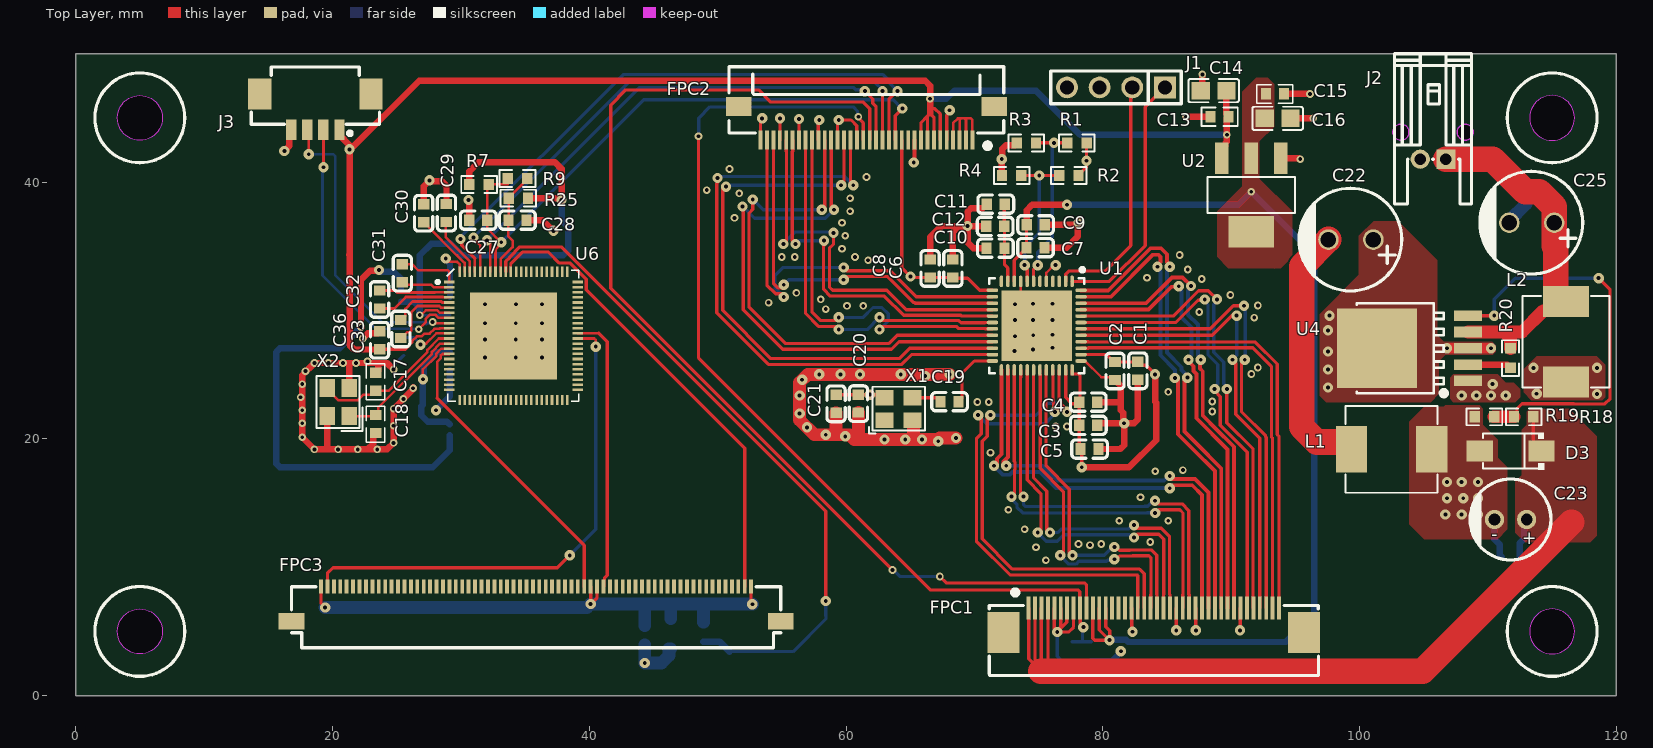
[diagram p0: Top Layer view]
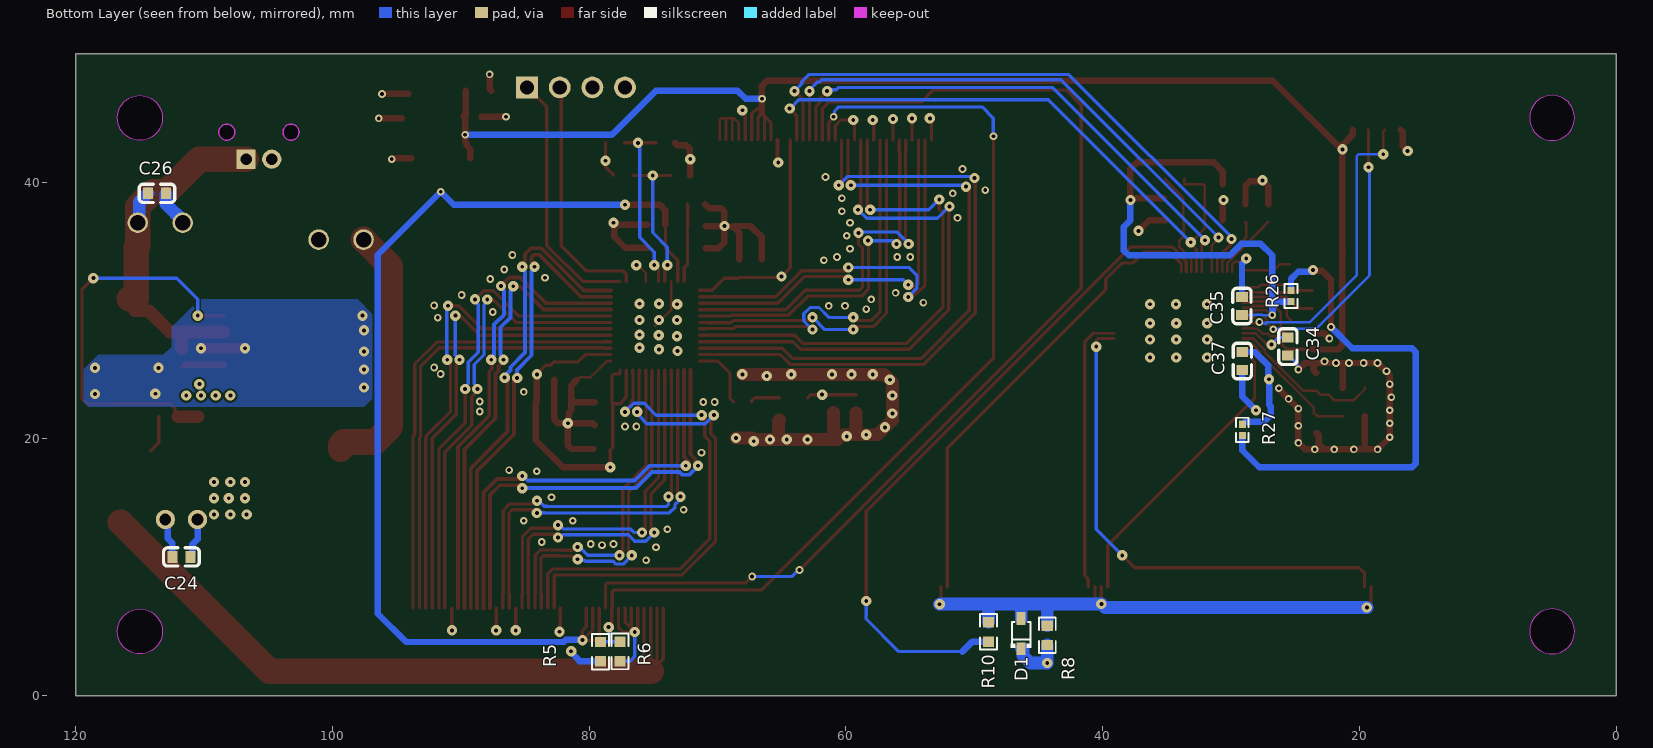
[diagram p1: Bottom Layer view, seen from below]
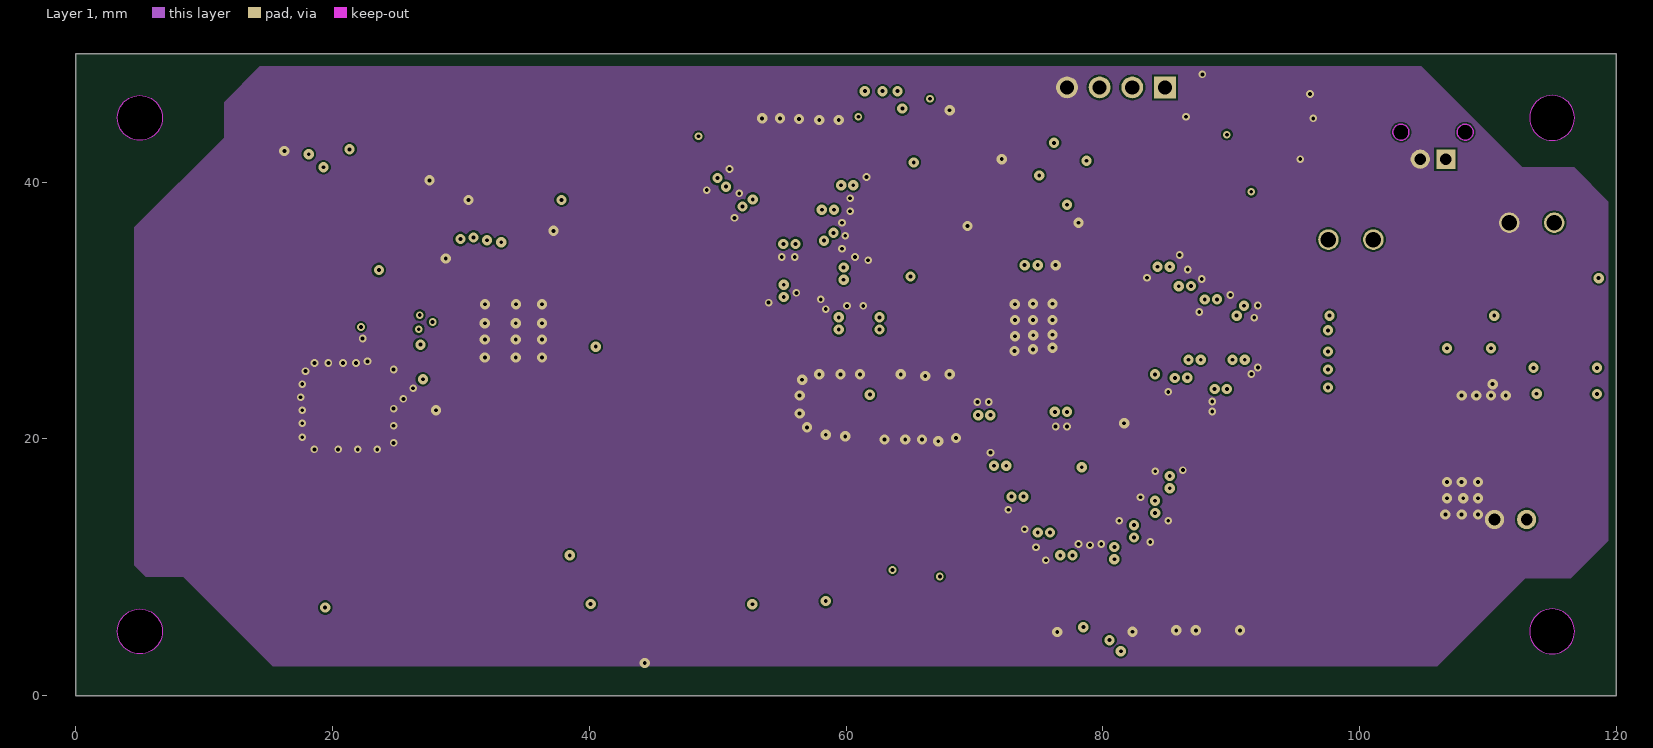
[diagram p2: Layer 1]
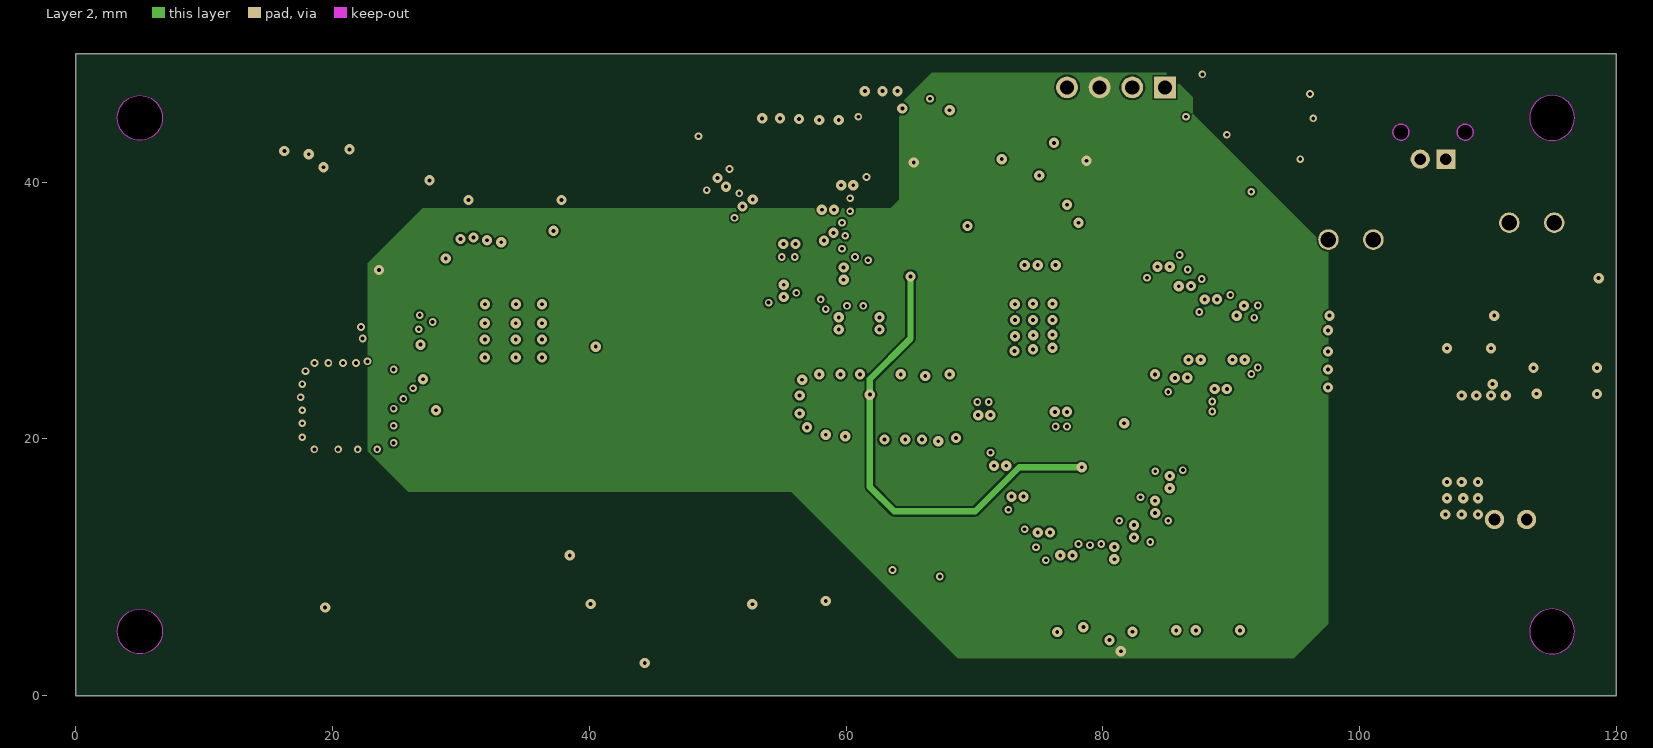
[diagram p3: Layer 2]
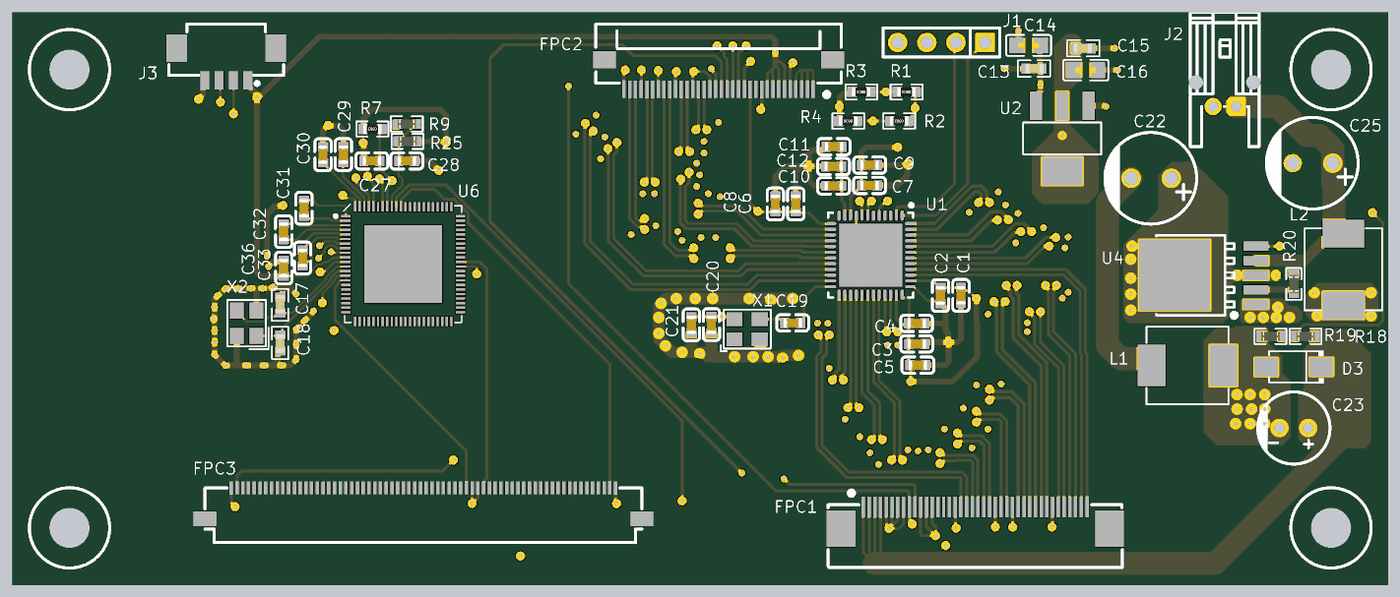
[diagram p4: 3D render of the assembled board from above, using the file's embedded part models]
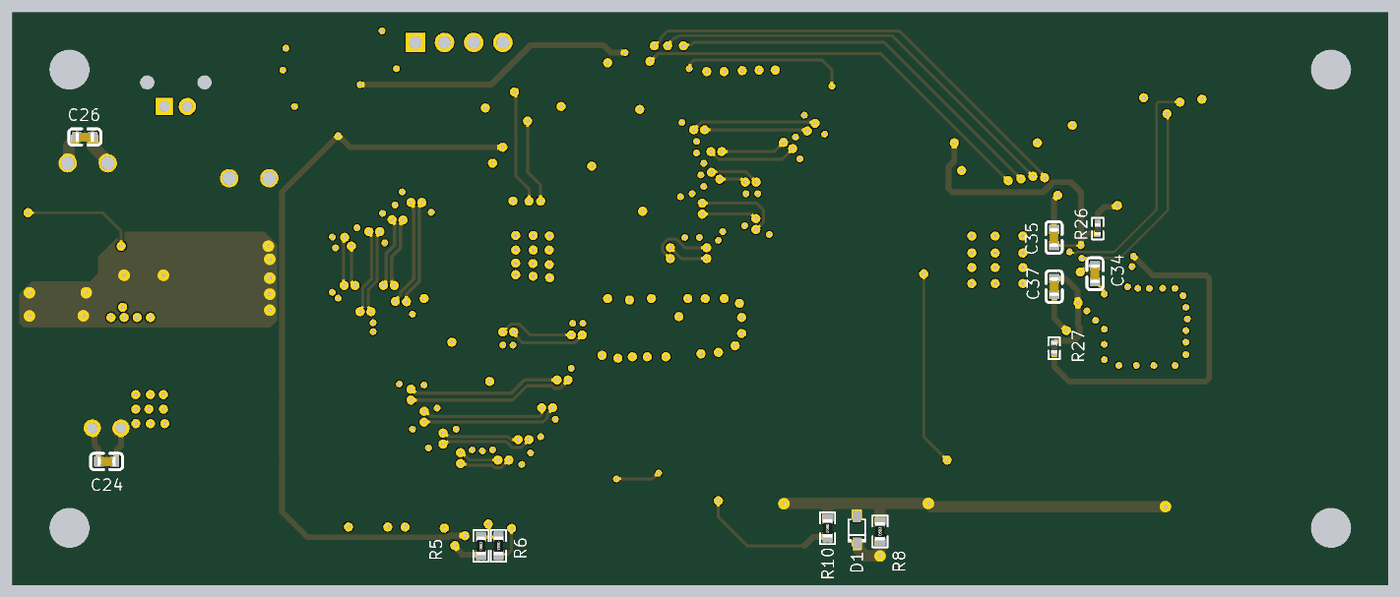
[diagram p5: 3D render of the assembled board from below, using the file's embedded part models]
# Altium PCB MISC71201-3.PcbDoc (part 1 of 3)
Units mm, origin at the board's own origin, x right, y up, seen from the top; angles counter-clockwise.
Board outline 120 x 50 mm, 4 copper layers (Top Layer, Layer 1, Layer 2, Bottom Layer), stack 0.603 mm thick; 69 components, 139 nets, 430 pads, 271 vias.

## Layer stack, top to bottom
Top Solder: solder mask 0.0102, Solder Resist, Dk 3.5
Top Layer: signal copper 0.0356
Dielectric 2: prepreg 0.0711, PP-006, Dk 4.1
Layer 1: signal copper 0.035
Dielectric 1: dielectric 0.32, FR-4, Dk 4.8
Layer 2: signal copper 0.035
Dielectric 3: prepreg 0.0711, PP-006, Dk 4.1
Bottom Layer: signal copper 0.0356
Bottom Solder: solder mask 0.0102, Solder Resist, Dk 3.5

## Board outline
0,0 120,0 120,50 0,50
cut-out: 113.25,45 ccw(c115,45) 115,43.25 ccw(c115,45) 116.75,45 ccw(c115,45) 115,46.75 ccw(c115,45)
cut-out: 113.25,5 ccw(c115,5) 115,3.25 ccw(c115,5) 116.75,5 ccw(c115,5) 115,6.75 ccw(c115,5)
cut-out: 5,3.25 cw(c5,5) 3.25,5 cw(c5,5) 5,6.75 cw(c5,5) 6.75,5 cw(c5,5)
cut-out: 5,43.25 cw(c5,45) 3.25,45 cw(c5,45) 5,46.75 cw(c5,45) 6.75,45 cw(c5,45)

## Design rules (kind name [scope] priority, off if disabled: settings)
Clearance [All] p1: gap=0.15 ignorepadtopadclearanceinfootprint=TRUE
ComponentClearance [All] p1: gap=0.01 collisioncheckmode=3 verticalgap=0.01 showdistances=FALSE
DiffPairsRouting DiffPairsRouting_14 [InDifferentialPair('MIPI_TD3')] p1: maxlimit=0.254 minlimit=0.2 mostfreqgap=0.2 toplayer_minwidth=0.15 toplayer_maxwidth=0.381 toplayer_prefwidth=0.3 midlayer1_minwidth=0.15 midlayer1_maxwidth=0.381 midlayer1_prefwidth=0.3 midlayer2_minwidth=0.15 midlayer2_maxwidth=0.381 midlayer2_prefwidth=0.3 bottomlayer_minwidth=0.15 bottomlayer_maxwidth=0.381 bottomlayer_prefwidth=0.3 maxuncoupledlength=12.7
DiffPairsRouting DiffPairsRouting_13 [InDifferentialPair('MIPI_TD2')] p2: maxlimit=0.254 minlimit=0.2 mostfreqgap=0.2 toplayer_minwidth=0.15 toplayer_maxwidth=0.381 toplayer_prefwidth=0.3 midlayer1_minwidth=0.15 midlayer1_maxwidth=0.381 midlayer1_prefwidth=0.3 midlayer2_minwidth=0.15 midlayer2_maxwidth=0.381 midlayer2_prefwidth=0.3 bottomlayer_minwidth=0.15 bottomlayer_maxwidth=0.381 bottomlayer_prefwidth=0.3 maxuncoupledlength=12.7
DiffPairsRouting DiffPairsRouting_12 [InDifferentialPair('MIPI_TD1')] p3: maxlimit=0.254 minlimit=0.2 mostfreqgap=0.2 toplayer_minwidth=0.15 toplayer_maxwidth=0.381 toplayer_prefwidth=0.3 midlayer1_minwidth=0.15 midlayer1_maxwidth=0.381 midlayer1_prefwidth=0.3 midlayer2_minwidth=0.15 midlayer2_maxwidth=0.381 midlayer2_prefwidth=0.3 bottomlayer_minwidth=0.15 bottomlayer_maxwidth=0.381 bottomlayer_prefwidth=0.3 maxuncoupledlength=12.7
DiffPairsRouting DiffPairsRouting_11 [InDifferentialPair('MIPI_TD0')] p4: maxlimit=0.254 minlimit=0.2 mostfreqgap=0.2 toplayer_minwidth=0.15 toplayer_maxwidth=0.381 toplayer_prefwidth=0.3 midlayer1_minwidth=0.15 midlayer1_maxwidth=0.381 midlayer1_prefwidth=0.3 midlayer2_minwidth=0.15 midlayer2_maxwidth=0.381 midlayer2_prefwidth=0.3 bottomlayer_minwidth=0.15 bottomlayer_maxwidth=0.381 bottomlayer_prefwidth=0.3 maxuncoupledlength=12.7
DiffPairsRouting DiffPairsRouting_10 [InDifferentialPair('MIPI_TC')] p5: maxlimit=0.254 minlimit=0.2 mostfreqgap=0.2 toplayer_minwidth=0.15 toplayer_maxwidth=0.381 toplayer_prefwidth=0.3 midlayer1_minwidth=0.15 midlayer1_maxwidth=0.381 midlayer1_prefwidth=0.3 midlayer2_minwidth=0.15 midlayer2_maxwidth=0.381 midlayer2_prefwidth=0.3 bottomlayer_minwidth=0.15 bottomlayer_maxwidth=0.381 bottomlayer_prefwidth=0.3 maxuncoupledlength=12.7
DiffPairsRouting DiffPairsRouting_9 [InDifferentialPair('RXOC')] p6: maxlimit=0.254 minlimit=0.2 mostfreqgap=0.2 toplayer_minwidth=0.15 toplayer_maxwidth=0.381 toplayer_prefwidth=0.3 midlayer1_minwidth=0.15 midlayer1_maxwidth=0.381 midlayer1_prefwidth=0.3 midlayer2_minwidth=0.15 midlayer2_maxwidth=0.381 midlayer2_prefwidth=0.3 bottomlayer_minwidth=0.15 bottomlayer_maxwidth=0.381 bottomlayer_prefwidth=0.3 maxuncoupledlength=12.7
DiffPairsRouting DiffPairsRouting_8 [InDifferentialPair('RXO3')] p7: maxlimit=0.254 minlimit=0.2 mostfreqgap=0.2 toplayer_minwidth=0.15 toplayer_maxwidth=0.381 toplayer_prefwidth=0.3 midlayer1_minwidth=0.15 midlayer1_maxwidth=0.381 midlayer1_prefwidth=0.3 midlayer2_minwidth=0.15 midlayer2_maxwidth=0.381 midlayer2_prefwidth=0.3 bottomlayer_minwidth=0.15 bottomlayer_maxwidth=0.381 bottomlayer_prefwidth=0.3 maxuncoupledlength=12.7
DiffPairsRouting DiffPairsRouting_7 [InDifferentialPair('RXO2')] p8: maxlimit=0.254 minlimit=0.2 mostfreqgap=0.2 toplayer_minwidth=0.15 toplayer_maxwidth=0.381 toplayer_prefwidth=0.3 midlayer1_minwidth=0.15 midlayer1_maxwidth=0.381 midlayer1_prefwidth=0.3 midlayer2_minwidth=0.15 midlayer2_maxwidth=0.381 midlayer2_prefwidth=0.3 bottomlayer_minwidth=0.15 bottomlayer_maxwidth=0.381 bottomlayer_prefwidth=0.3 maxuncoupledlength=12.7
DiffPairsRouting DiffPairsRouting_6 [InDifferentialPair('RXO1')] p9: maxlimit=0.254 minlimit=0.2 mostfreqgap=0.2 toplayer_minwidth=0.15 toplayer_maxwidth=0.381 toplayer_prefwidth=0.3 midlayer1_minwidth=0.15 midlayer1_maxwidth=0.381 midlayer1_prefwidth=0.3 midlayer2_minwidth=0.15 midlayer2_maxwidth=0.381 midlayer2_prefwidth=0.3 bottomlayer_minwidth=0.15 bottomlayer_maxwidth=0.381 bottomlayer_prefwidth=0.3 maxuncoupledlength=12.7
DiffPairsRouting DiffPairsRouting_5 [InDifferentialPair('RXO0')] p10: maxlimit=0.254 minlimit=0.2 mostfreqgap=0.2 toplayer_minwidth=0.15 toplayer_maxwidth=0.381 toplayer_prefwidth=0.3 midlayer1_minwidth=0.15 midlayer1_maxwidth=0.381 midlayer1_prefwidth=0.3 midlayer2_minwidth=0.15 midlayer2_maxwidth=0.381 midlayer2_prefwidth=0.3 bottomlayer_minwidth=0.15 bottomlayer_maxwidth=0.381 bottomlayer_prefwidth=0.3 maxuncoupledlength=12.7
DiffPairsRouting DiffPairsRouting_4 [InDifferentialPair('RXEC')] p11: maxlimit=0.254 minlimit=0.2 mostfreqgap=0.2 toplayer_minwidth=0.15 toplayer_maxwidth=0.381 toplayer_prefwidth=0.3 midlayer1_minwidth=0.15 midlayer1_maxwidth=0.381 midlayer1_prefwidth=0.3 midlayer2_minwidth=0.15 midlayer2_maxwidth=0.381 midlayer2_prefwidth=0.3 bottomlayer_minwidth=0.15 bottomlayer_maxwidth=0.381 bottomlayer_prefwidth=0.3 maxuncoupledlength=12.7
DiffPairsRouting DiffPairsRouting_3 [InDifferentialPair('RXE3')] p12: maxlimit=0.254 minlimit=0.2 mostfreqgap=0.2 toplayer_minwidth=0.15 toplayer_maxwidth=0.381 toplayer_prefwidth=0.3 midlayer1_minwidth=0.15 midlayer1_maxwidth=0.381 midlayer1_prefwidth=0.3 midlayer2_minwidth=0.15 midlayer2_maxwidth=0.381 midlayer2_prefwidth=0.3 bottomlayer_minwidth=0.15 bottomlayer_maxwidth=0.381 bottomlayer_prefwidth=0.3 maxuncoupledlength=12.7
DiffPairsRouting DiffPairsRouting_2 [InDifferentialPair('RXE2')] p13: maxlimit=0.254 minlimit=0.2 mostfreqgap=0.2 toplayer_minwidth=0.15 toplayer_maxwidth=0.381 toplayer_prefwidth=0.3 midlayer1_minwidth=0.15 midlayer1_maxwidth=0.381 midlayer1_prefwidth=0.3 midlayer2_minwidth=0.15 midlayer2_maxwidth=0.381 midlayer2_prefwidth=0.3 bottomlayer_minwidth=0.15 bottomlayer_maxwidth=0.381 bottomlayer_prefwidth=0.3 maxuncoupledlength=12.7
DiffPairsRouting DiffPairsRouting_1 [InDifferentialPair('RXE1')] p14: maxlimit=0.254 minlimit=0.2 mostfreqgap=0.2 toplayer_minwidth=0.15 toplayer_maxwidth=0.381 toplayer_prefwidth=0.3 midlayer1_minwidth=0.15 midlayer1_maxwidth=0.381 midlayer1_prefwidth=0.3 midlayer2_minwidth=0.15 midlayer2_maxwidth=0.381 midlayer2_prefwidth=0.3 bottomlayer_minwidth=0.15 bottomlayer_maxwidth=0.381 bottomlayer_prefwidth=0.3 maxuncoupledlength=12.7
DiffPairsRouting [InDifferentialPair('RXE0')] p15: maxlimit=0.254 minlimit=0.2 mostfreqgap=0.2 toplayer_minwidth=0.15 toplayer_maxwidth=0.3 toplayer_prefwidth=0.3 midlayer1_minwidth=0.15 midlayer1_maxwidth=0.3 midlayer1_prefwidth=0.3 midlayer2_minwidth=0.15 midlayer2_maxwidth=0.3 midlayer2_prefwidth=0.3 bottomlayer_minwidth=0.15 bottomlayer_maxwidth=0.3 bottomlayer_prefwidth=0.3 maxuncoupledlength=12.7
MinimumSolderMaskSliver [All] p1: minsoldermaskwidth=0.01
PlaneConnect [All] p1: planeconnectstyle=Direct reliefexpansion=0.508 reliefentries=4 reliefconductorwidth=0.254 reliefairgap=0.254
PolygonConnect [All] p1: connectstyle=Direct reliefconductorwidth=0.254 reliefentries=4 polygonreliefangle="90 Angle" airgapwidth=0.254
RoutingVias [All] p1: holewidth=0.3 width=0.8 viastyle="Through Hole" minholewidth=0.3 minwidth=0.8 maxholewidth=0.711 maxwidth=1.27
SilkToSilkClearance [All] p1: silktosilkclearance=0.01
SilkToSolderMaskClearance [IsPad] p1: minsilkscreentomaskgap=0.01 clearancetoexposedcopper=TRUE
SolderMaskExpansion [All] p1: expansion=0.102 istentingtop=FALSE
Width [All] p1: maxlimit=2 minlimit=0.18 preferedwidth=0.2
24 further rules are at their usual default settings.

## Classes and differential pairs
component class Sheet2: C17 C18 C27 C28 C29 C30 C31 C32 C33 C34 C35 C36 C37 D1 FPC3 J3 R7 R8 R9 R10 R25 R26 R27 U6 X2
component class Sheet1: C1 C2 C3 C4 C5 C6 C7 C8 C9 C10 C11 C12 C13 C14 C15 C16 C19 C20 C21 C22 C23 C24 C25 C26 D3 FPC1 FPC2 J1 J2 J? L1 L2 R1 R2 R3 R4 R5 R6 R18 R19 R20 U1 U2 U4 X1
differential pair MIPI_TD3: +MIPI_TD3_P -MIPI_TD3_N
differential pair MIPI_TD2: +MIPI_TD2_P -MIPI_TD2_N
differential pair MIPI_TD1: +MIPI_TD1_P -MIPI_TD1_N
differential pair MIPI_TD0: +MIPI_TD0_P -MIPI_TD0_N
differential pair MIPI_TC: +MIPI_TC_P -MIPI_TC_N
differential pair RXOC: +RXOC_P -RXOC_N
differential pair RXO3: +RXO3_P -RXO3_N
differential pair RXO2: +RXO2_P -RXO2_N
differential pair RXO1: +RXO1_P -RXO1_N
differential pair RXO0: +RXO0_P -RXO0_N
differential pair RXEC: +RXEC_P -RXEC_N
differential pair RXE3: +RXE3_P -RXE3_N
differential pair RXE2: +RXE2_P -RXE2_N
differential pair RXE1: +RXE1_P -RXE1_N
differential pair RXE0: +RXE0_P -RXE0_N

## Components (designator, comment, footprint, x,y, rotation, side; value= is the part's Value field where it differs from the comment)
C1 "cc0603krx7r0bb103" C0603 82.728,25.296 r90 top value=10nF
C2 "cc0603krx7r0bb103" C0603 80.95,25.281 r90 top value=10nF
C3 "cc0603krx7r0bb104" C0603 78.875,21.052 r180 top value=100nF
C4 "cc0603krx7r0bb104" C0603 78.869,22.85 r180 top value=100nF
C5 "cc0603krx7r8bb105" C0603 78.971,19.207 r0 top value=1uF
C6 "cc0603krx7r0bb103" C0603 68.326,33.274 r270 top value=10nF
C7 "cc0603krx7r0bb103" C0603 74.756,34.89 r180 top value=10nF
C8 "cc0603krx7r0bb104" C0603 66.548,33.274 r270 top value=100nF
C9 "cc0603krx7r0bb104" C0603 74.771,36.668 r180 top value=100nF
C10 "cc0603krx7r0bb103" C0603 71.636,34.851 r0 top value=10nF
C11 "cc0603krx7r0bb104" C0603 71.666,38.28 r0 top value=100nF
C12 "cc0603krx7r8bb105" C0603 71.62,36.546 r180 top value=1uF
C13 "100nF 50V 0603" "CAP C0603" 89.789,45.085 r180 top
C14 "10uF 25V 0805" "CAP C0805" 87.63,47.117 r0 top
C15 "100nF 50V 0603" "CAP C0603" 92.71,46.863 r0 top
C16 "10uF 25V 0805" "CAP C0805" 94.615,44.958 r180 top
C17 "CC0603JRNPO9BN120" "CAP C0603" 23.368,25.146 r270 top
C18 "CC0603JRNPO9BN120" "CAP C0603" 23.368,20.447 r90 top
C19 "cc0603krx7r9bb102" C0603 68.064,22.893 r180 top value=1nF
C20 "cc0603krx7r0bb103" C0603 60.97,22.741 r90 top value=10nF
C21 "cc0603krx7r0bb104" C0603 59.224,22.725 r90 top value=100nF
C22 "era63v100m8x12" CAP-TH_BD8.0-P3.50-D0.8-FD 99.325,35.518 r180 top value=100uF
C23 "erg25v220m6x11" CAP-TH_BD6.3-P2.50-D0.5-FD 111.76,13.716 r180 top value=220uF
C24 "cc0603krx7r0bb104" C0603 111.76,10.795 r0 bottom value=100nF
C25 "era63v100m8x12" CAP-TH_BD8.0-P3.50-D0.8-FD 113.411,36.83 r180 top value=100uF
C26 "cc0603krx7r0bb104" C0603 113.665,39.116 r0 bottom value=100nF
C27 "0.1u X7R 10% 6.3V" C0603 31.361,37.031 r180 top
C28 "2.2u X7R 10% 6.3V" C0603 34.409,37.031 r180 top
C29 "1u X7R 10% 50V" C0603 28.882,37.584 r270 top
C30 "1u X7R 10% 50V" C0603 27.104,37.569 r270 top
C31 "1u X7R 10% 50V" C0603 25.446,32.901 r270 top
C32 "1u X7R 10% 50V" C0603 23.675,30.853 r270 top
C33 "1u X7R 10% 50V" C0603 25.326,28.552 r270 top
C34 "1u X7R 10% 6.3V" C0603 25.58,27.186 r90 bottom
C35 "1u X7R 10% 6.3V" C0603 29.157,30.345 r270 bottom
C36 "1u X7R 10% 6.3V" C0603 23.675,27.678 r270 top
C37 "1u X7R 10% 6.3V" C0603 29.136,26.058 r90 bottom
D1 "pdyl240b" SOD-323_L1.8-W1.3-LS2.5-RD 46.355,4.826 r90 bottom
D3 "ss34" SMA_L4.3-W2.6-LS5.0-RD 111.76,19.05 r180 top
FPC1 "fc-05d40p11h20" FPC-SMD_40P-P0.50_FC-05D40P11H20 83.976,5.875 r0 top
FPC2 "fc-05a34p011h20" FPC-SMD_FC-05A34P011H20 61.595,44.577 r180 top
FPC3 "afc18-s68fia-00" CONN-SMD_AFC18-S68FIA-00 35.86,7.134 r0 top
J1 "hx pz2.54-1x4p zz" HDR-TH_4P-P2.54-V-M 81.026,47.371 r180 top
J2 "s02b-pask-2(lf)(sn)" CONN-TH_S02B-PASK-2-LF-SN 105.724,41.783 r0 top
J3 "mx1.25mm-4p-wt" CONN-SMD_MX1.25MM-4P-WT 18.669,45.466 r180 top
L1 "fxl0630-150-m" IND-SMD_L7.0-W6.6_FXL0630 102.489,19.177 r180 top
L2 "fxl0630-150-m" IND-SMD_L7.0-W6.6_FXL0630 116.078,27.559 r270 top
R1 "10K 0603 1%" "RES R0603" 78.74,43.053 r180 top
R2 "10K 0603 1%" "RES R0603" 78.105,40.513 r180 top
R3 "10K 0603 1%" "RES R0603" 74.803,43.053 r180 top
R4 "10K 0603 1%" "RES R0603" 73.66,40.513 r180 top
R5 "10K 0603 1%" "RES R0603" 79.121,2.667 r90 bottom
R6 "10K 0603 1%" "RES R0603" 77.597,4.191 r270 bottom
R7 "10K 0603 1% NC" "RES R0603" 32.171,39.818 r180 top
R8 "0R 0603" "RES R0603" 44.323,3.937 r90 bottom value=0R
R9 "0R 5% NC" R0603 34.417,40.259 r180 top value=10K
R10 "0R 0603" "RES R0603" 48.895,5.715 r270 bottom value=330R
R18 "rt0603brd0786k6l" R0603 112.776,21.717 r0 top value=86.6kΩ
R19 "rt0603brd0710kl" R0603 109.728,21.717 r180 top value=10kΩ
R20 "rt0603brd0710kl" R0603 111.76,26.289 r90 top value=10kΩ
R25 "0R 5%" R0603 34.478,38.738 r0 top value=10K
R26 "0R 5%" R0402 25.342,31.12 r270 bottom
R27 "0R 5%" R0402 29.134,20.696 r90 bottom
U1 "GM8775C" UFQFPN-48_L7.0-W7.0-P0.50-BL-EP 74.857,28.811 r180 top
U2 "bl1117-33cx" SOT-223_L6.5-W3.5-P2.30-LS7.0-BR 91.567,38.989 r90 top
U4 "xl6008e1" TO-252-5_L6.6-W5.8-P1.27-TL 104.902,27.051 r180 top
U6 "ILI2511/QFN-88/10X10" ILI2511/QFN-88/10X10 29.101,32.215 r0 top
X1 "ot322526mjba4sl" OSC-SMD_4P-L3.2-W2.5-BL 64.084,22.333 r0 top value=26MHz
X2 "x322512msb4si" CRYSTAL-SMD_4P-L3.2-W2.5-BL 20.447,22.86 r90 top value=12MHz

## Footprints (in the part's own frame and the unit in brackets; to place one, negate y for a bottom-side part, rotate by r counter-clockwise, add the part's x,y. Pads: shape width x height; smd on the part's side, far side on the other; paste and mask are expansions set on the pad)
C0603 [mil]
  rect 31.5x35.4 smd: 1(-27.5,0) 2(27.6,0)
  silkscreen extent -55,-28 55,28, body extent -31,-16 31,16, height 16
"CAP C0603" [mm]
  rect 0.8x0.9 smd: 1(0,0) 2(1.4,0)
  silkscreen extent -0.72,-0.72 2.1,0.72, body extent -0.17,-0.4 1.44,0.4, height 0.8
"CAP C0805" [mm]
  rect 1.41x1.35 smd paste-100 mask+0.051: 1(0,0) 2(2,0)
  silkscreen extent -0.96,-0.9 2.96,0.9, body extent 0.02,-0.63 2.02,0.63, height 0.6
CAP-TH_BD6.3-P2.50-D0.5-FD [mm]
  round 1.5 hole 0.9 paste-2539.97 mask+0.05: 1(-1.25,0) 2(1.25,0)
  silkscreen extent -3.15,-3.15 3.21,3.15
CAP-TH_BD8.0-P3.50-D0.8-FD [mm]
  round 1.6 hole 1.2 paste-2539.97 mask+0.05: 1(-1.75,0) 2(1.75,0)
  silkscreen extent -3.96,-4 4.04,4
CONN-SMD_AFC18-S68FIA-00 [mm]
  rect 0.3x1.1 smd paste+0 mask+0.05: 1(-16.75,1.35) 2(-16.25,1.35) 3(-15.75,1.35) 4(-15.25,1.35) 5(-14.75,1.35) 6(-14.25,1.35) 7(-13.75,1.35) 8(-13.25,1.35) 9(-12.75,1.35) 10(-12.25,1.35) 11(-11.75,1.35) 12(-11.25,1.35) 13(-10.75,1.35) 14(-10.25,1.35) 15(-9.75,1.35) 16(-9.25,1.35) 17(-8.75,1.35) 18(-8.25,1.35) 19(-7.75,1.35) 20(-7.25,1.35) 21(-6.75,1.35) 22(-6.25,1.35) 23(-5.75,1.35) 24(-5.25,1.35) 25(-4.75,1.35) 26(-4.25,1.35) 27(-3.75,1.35) 28(-3.25,1.35) 29(-2.75,1.35) 30(-2.25,1.35) 31(-1.75,1.35) 32(-1.25,1.35) 33(-0.75,1.35) 34(-0.25,1.35) 35(0.25,1.35) 36(0.75,1.35) 37(1.25,1.35) 38(1.75,1.35) 39(2.25,1.35) 40(2.75,1.35) 41(3.25,1.35) 42(3.75,1.35) 43(4.25,1.35) 44(4.75,1.35) 45(5.25,1.35) 46(5.75,1.35) 47(6.25,1.35) 48(6.75,1.35) 49(7.25,1.35) 50(7.75,1.35) 51(8.25,1.35) 52(8.75,1.35) 53(9.25,1.35) 54(9.75,1.35) 55(10.25,1.35) 56(10.75,1.35) 57(11.25,1.35) 58(11.75,1.35) 59(12.25,1.35) 60(12.75,1.35) 61(13.25,1.35) 62(13.75,1.35) 63(14.25,1.35) 64(14.75,1.35) 65(15.25,1.35) 66(15.75,1.35) 67(16.25,1.35) 68(16.75,1.35)
  rect 2x1.3 smd paste+0 mask+0.05: 69(19.05,-1.35) 70(-19.05,-1.35)
  silkscreen extent -19.05,-3.4 19.05,1.35
CONN-SMD_MX1.25MM-4P-WT [mm]
  rect 0.8x1.6 smd paste+0 mask+0.05: 1(-1.875,1.4) 2(-0.625,1.4) 3(0.625,1.4) 4(1.875,1.4)
  rect 1.8x2.4 smd paste+0 mask+0.05: 5(4.325,-1.4) 6(-4.325,-1.4)
  silkscreen extent -5,-3.5 5,1.82
CONN-TH_S02B-PASK-2-LF-SN [mm]
  rect 1.5x1.5 hole 0.9: 1(1,0)
  round 1.5 hole 0.9: 2(-1,0)
  Keep-Out Layer board cut-out: -1.875,2.1 -1.875,1.976 -1.97,1.746 -2.146,1.57 -2.376,1.475 -2.624,1.475 -2.854,1.57 -3.03,1.746 -3.125,1.976 -3.125,2.1 -3.125,2.224 -3.03,2.454 -2.854,2.63 -2.624,2.725 -2.376,2.725 -2.146,2.63 -1.97,2.454 -1.875,2.224 -1.875,2.1 -1.875,2.1
  Keep-Out Layer board cut-out: 3.125,2.1 3.125,1.976 3.03,1.746 2.854,1.57 2.624,1.475 2.376,1.475 2.146,1.57 1.97,1.746 1.875,1.976 1.875,2.1 1.875,2.224 1.97,2.454 2.146,2.63 2.376,2.725 2.624,2.725 2.854,2.63 3.03,2.454 3.125,2.224 3.125,2.1 3.125,2.1
  Keep-Out Layer circle w0.003: c-2.5,2.1 r0.625
  Keep-Out Layer circle w0.003: c2.5,2.1 r0.625
  Keep-Out Layer region: -1.875,2.1 -1.884,1.992 -1.913,1.886 -1.959,1.788 -2.021,1.698 -2.098,1.621 -2.187,1.559 -2.286,1.513 -2.391,1.485 -2.5,1.475 -2.608,1.485 -2.714,1.513 -2.812,1.559 -2.902,1.621 -2.979,1.698 -3.041,1.788 -3.087,1.886 -3.115,1.992 -3.125,2.1 -3.115,2.209 -3.087,2.314 -3.041,2.413 -2.979,2.502 -2.902,2.579 -2.812,2.641 -2.714,2.687 -2.608,2.716 -2.5,2.725 -2.391,2.716 -2.286,2.687 -2.187,2.641 -2.098,2.579 -2.021,2.502 -1.959,2.413 -1.913,2.314 -1.884,2.209 -1.875,2.1
  Keep-Out Layer region: -1.875,2.1 -1.875,1.976 -1.97,1.746 -2.146,1.57 -2.376,1.475 -2.624,1.475 -2.854,1.57 -3.03,1.746 -3.125,1.976 -3.125,2.1 -3.125,2.224 -3.03,2.454 -2.854,2.63 -2.624,2.725 -2.376,2.725 -2.146,2.63 -1.97,2.454 -1.875,2.224 -1.875,2.1 -1.875,2.1
  Keep-Out Layer region: 3.125,2.1 3.116,1.992 3.087,1.886 3.041,1.788 2.979,1.698 2.902,1.621 2.813,1.559 2.714,1.513 2.609,1.485 2.5,1.475 2.392,1.485 2.286,1.513 2.188,1.559 2.098,1.621 2.021,1.698 1.959,1.788 1.913,1.886 1.885,1.992 1.875,2.1 1.885,2.209 1.913,2.314 1.959,2.413 2.021,2.502 2.098,2.579 2.188,2.641 2.286,2.687 2.392,2.716 2.5,2.725 2.609,2.716 2.714,2.687 2.813,2.641 2.902,2.579 2.979,2.502 3.041,2.413 3.087,2.314 3.116,2.209 3.125,2.1
  Keep-Out Layer region: 3.125,2.1 3.125,1.976 3.03,1.746 2.854,1.57 2.624,1.475 2.376,1.475 2.146,1.57 1.97,1.746 1.875,1.976 1.875,2.1 1.875,2.224 1.97,2.454 2.146,2.63 2.376,2.725 2.624,2.725 2.854,2.63 3.03,2.454 3.125,2.224 3.125,2.1 3.125,2.1
  silkscreen extent -3,-3.5 3,8.2
CRYSTAL-SMD_4P-L3.2-W2.5-BL [mm]
  rect 1.4x1.2 smd: 1(-1.1,-0.85) 2(1.1,-0.85) 3(1.1,0.85) 4(-1.1,0.85)
  silkscreen extent -2.26,-1.91 2.03,1.68
FPC-SMD_40P-P0.50_FC-05D40P11H20 [mm]
  rect 0.3x1.8 smd paste+0 mask+0.05: 1(-9.75,0.95) 2(-9.25,0.95) 3(-8.75,0.95) 4(-8.25,0.95) 5(-7.75,0.95) 6(-7.25,0.95) 7(-6.75,0.95) 8(-6.25,0.95) 9(-5.75,0.95) 10(-5.25,0.95) 11(-4.75,0.95) 12(-4.25,0.95) 13(-3.75,0.95) 14(-3.25,0.95) 15(-2.75,0.95) 16(-2.25,0.95) 17(-1.75,0.95) 18(-1.25,0.95) 19(-0.75,0.95) 20(-0.25,0.95) 21(0.25,0.95) 22(0.75,0.95) 23(1.25,0.95) 24(1.75,0.95) 25(2.25,0.95) 26(2.75,0.95) 27(3.25,0.95) 28(3.75,0.95) 29(4.25,0.95) 30(4.75,0.95) 31(5.25,0.95) 32(5.75,0.95) 33(6.25,0.95) 34(6.75,0.95) 35(7.25,0.95) 36(7.75,0.95) 37(8.25,0.95) 38(8.75,0.95) 39(9.25,0.95) 40(9.75,0.95)
  rect 2.5x3.2 smd paste+0 mask+0.05: 41(11.7,-0.95) 42(-11.7,-0.95)
  silkscreen extent -12.83,-4.32 12.83,2.36
FPC-SMD_FC-05A34P011H20 [mm]
  rect 0.3x1.5 smd paste+0 mask+0.051: 1(8.25,1.3) 2(7.75,1.3) 3(7.25,1.3) 4(6.75,1.3) 5(6.25,1.3) 6(5.75,1.3) 7(5.25,1.3) 8(4.75,1.3) 9(4.25,1.3) 10(3.75,1.3) 11(3.25,1.3) 12(2.75,1.3) 13(2.25,1.3) 14(1.75,1.3) 15(1.25,1.3) 16(0.75,1.3) 17(0.25,1.3) 18(-0.25,1.3) 19(-0.75,1.3) 20(-1.25,1.3) 21(-1.75,1.3) 22(-2.25,1.3) 23(-2.75,1.3) 24(-3.25,1.3) 25(-3.75,1.3) 26(-4.25,1.3) 27(-4.75,1.3) 28(-5.25,1.3) 29(-5.75,1.3) 30(-6.25,1.3) 31(-6.75,1.3) 32(-7.25,1.3) 33(-7.75,1.3) 34(-8.25,1.3)
  rect 2x1.5 smd paste+0 mask+0.051: 35(9.95,-1.3) 36(-9.95,-1.3)
  silkscreen extent -10.7,-4.4 10.7,2.16
HDR-TH_4P-P2.54-V-M [mm]
  rect 1.699x1.699 hole 1.1: 1(-3.81,0)
  round 1.699 hole 1.1: 2(-1.27,0) 3(1.27,0) 4(3.81,0)
  silkscreen extent -5.08,-1.27 5.08,1.27
ILI2511/QFN-88/10X10 [mm]
  rect 0.8x0.2 smd: 1(0,0) 2(0,-0.4) 3(0,-0.8) 4(0,-1.2) 5(0,-1.6) 6(0,-2) 7(0,-2.4) 8(0,-2.8) 9(0,-3.2) 10(0,-3.6) 11(0,-4) 12(0,-4.4) 13(0,-4.8) 14(0,-5.2) 15(0,-5.6) 16(0,-6) 17(0,-6.4) 18(0,-6.8) 19(0,-7.2) 20(0,-7.6) 21(0,-8) 22(0,-8.4) 45(10,-8.4) 46(10,-8) 47(10,-7.6) 48(10,-7.2) 49(10,-6.8) 50(10,-6.4) 51(10,-6) 52(10,-5.6) 53(10,-5.2) 54(10,-4.8) 55(10,-4.4) 56(10,-4) 57(10,-3.6) 58(10,-3.2) 59(10,-2.8) 60(10,-2.4) 61(10,-2) 62(10,-1.6) 63(10,-1.2) 64(10,-0.8) 65(10,-0.4) 66(10,0)
  rect 0.2x0.8 smd: 23(0.8,-9.2) 24(1.2,-9.2) 25(1.6,-9.2) 26(2,-9.2) 27(2.4,-9.2) 28(2.8,-9.2) 29(3.2,-9.2) 30(3.6,-9.2) 31(4,-9.2) 32(4.4,-9.2) 33(4.8,-9.2) 34(5.2,-9.2) 35(5.6,-9.2) 36(6,-9.2) 37(6.4,-9.2) 38(6.8,-9.2) 39(7.2,-9.2) 40(7.6,-9.2) 41(8,-9.2) 42(8.4,-9.2) 43(8.8,-9.2) 44(9.2,-9.2) 67(9.2,0.8) 68(8.8,0.8) 69(8.4,0.8) 70(8,0.8) 71(7.6,0.8) 72(7.2,0.8) 73(6.8,0.8) 74(6.4,0.8) 75(6,0.8) 76(5.6,0.8) 77(5.2,0.8) 78(4.8,0.8) 79(4.4,0.8) 80(4,0.8) 81(3.6,0.8) 82(3.2,0.8) 83(2.8,0.8) 84(2.4,0.8) 85(2,0.8) 86(1.6,0.8) 87(1.2,0.8) 88(0.8,0.8)
  rect 6.8x6.8 smd: 89(5,-4.2)
  silkscreen extent -1.02,-9.3 10.1,1.03
IND-SMD_L7.0-W6.6_FXL0630 [mm]
  rect 2.424x3.62 smd: 1(3.128,0) 2(-3.128,0)
  silkscreen extent -3.58,-3.38 3.58,3.38
OSC-SMD_4P-L3.2-W2.5-BL [mm]
  rect 1.4x1.2 smd: 1(-1.1,-0.875) 2(1.1,-0.875) 3(1.1,0.875) 4(-1.1,0.875)
  silkscreen extent -2.29,-1.9 2.07,1.72
R0402 [mil]
  rect 22.3x21.3 smd paste-3937 mask+2: 1(-17.1,0) 2(17,0)
  silkscreen extent -37,-20 37,20, body extent -19,-10 23,10, height 28
R0603 [mil]
  rect 31.8x34 smd: 1(-29.6,0) 2(29.7,0)
  silkscreen extent -54,-26 55,26, body extent -32,-16 32,16, height 17
"RES R0603" [mm]
  rect 0.806x0.864 smd paste-100: 1(0,0) 2(1.507,0)
  silkscreen extent -0.63,-0.66 2.14,0.66, body extent -0.04,-0.4 1.56,0.4, height 0.43
SMA_L4.3-W2.6-LS5.0-RD [mm]
  rect 2.047x1.621 smd: 1(-2.403,-0.01) 2(2.405,0.01)
  silkscreen extent -2.61,-1.44 2.17,1.44
SOD-323_L1.8-W1.3-LS2.5-RD [mm]
  rect 1.001x0.701 smd: 1(-1.171,0) 2(1.173,0)
  silkscreen extent -1.08,-0.8 0.9,0.8
SOT-223_L6.5-W3.5-P2.30-LS7.0-BR [mm]
  rect 2.465x1.05 smd: 1(2.857,-2.3) 2(2.857,0) 3(2.857,2.3)
  rect 2.465x3.54 smd: 4(-2.857,0)
  silkscreen extent -1.4,-3.4 1.4,3.4
TO-252-5_L6.6-W5.8-P1.27-TL [mil]
  rect 86.61x32.5 smd: 1(-139.5,100) 2(-139.5,50) 3(-139.5,0) 4(-139.5,-50) 5(-139.5,-100)
  rect 244.5x244.5 smd: 6(139.5,0)
  silkscreen extent -73,-138 202,146
UFQFPN-48_L7.0-W7.0-P0.50-BL-EP [mm]
  oval 0.28x0.9 smd: 1(-2.751,-3.449) 2(-2.25,-3.449) 3(-1.75,-3.449) 4(-1.25,-3.449) 5(-0.749,-3.449) 6(-0.249,-3.449) 7(0.249,-3.449) 8(0.749,-3.449) 9(1.25,-3.449) 10(1.75,-3.449) 11(2.251,-3.449) 12(2.751,-3.449) 25(2.751,3.449) 26(2.251,3.449) 27(1.75,3.449) 28(1.25,3.449) 29(0.749,3.449) 30(0.249,3.449) 31(-0.249,3.449) 32(-0.749,3.449) 33(-1.25,3.449) 34(-1.75,3.449) 35(-2.25,3.449) 36(-2.751,3.449)
  oval 0.9x0.28 smd: 13(3.449,-2.751) 14(3.449,-2.251) 15(3.449,-1.75) 16(3.449,-1.25) 17(3.449,-0.749) 18(3.449,-0.249) 19(3.449,0.249) 20(3.449,0.749) 21(3.449,1.25) 22(3.449,1.75) 23(3.449,2.25) 24(3.449,2.751) 37(-3.449,2.751) 38(-3.449,2.25) 39(-3.449,1.75) 40(-3.449,1.25) 41(-3.449,0.749) 42(-3.449,0.249) 43(-3.449,-0.249) 44(-3.449,-0.749) 45(-3.449,-1.25) 46(-3.449,-1.75) 47(-3.449,-2.251) 48(-3.449,-2.751)
  rect 5.5x5.5 smd: 49(0,0)
  silkscreen extent -3.7,-4.5 3.7,3.7

## Part data
C1 C2 C6 C7 C10 C20: "Capacitance:10nF;Tolerance:±10%;Rated voltage:100V;Temp. coefficient:X7R;", JLCPCB Part Class="Extended Part", LCSC Part Name="10nF ±10% 100V", Manufacturer=YAGEO(国巨), ManufacturerPart=CC0603KRX7R0BB103, Temperature Coefficient=X7R, Tolerance=±10%, Voltage Rating=100V
C3 C4 C8 C9 C11 C21 C24 C26: "Capacitance:100nF;Tolerance:±10%;Rated voltage:100V;Temp. coefficient:X7R;", JLCPCB Part Class="Extended Part", LCSC Part Name="100nF ±10% 100V", Manufacturer=YAGEO(国巨), ManufacturerPart=CC0603KRX7R0BB104, Temperature Coefficient=X7R, Tolerance=±10%, Voltage Rating=100V
C5 C12: "Capacitance:1uF;Tolerance:±10%;Rated voltage:25V;Temp. coefficient:X7R;", JLCPCB Part Class="Extended Part", LCSC Part Name="1uF ±10% 25V", Manufacturer=YAGEO(国巨), ManufacturerPart=CC0603KRX7R8BB105, Temperature Coefficient=X7R, Tolerance=±10%, Voltage Rating=25V
C13 C14 C15 C16: library part "CAPACITOR CER"
C17 C18: "12PF"
C19: "Capacitance:1nF;Tolerance:±10%;Rated voltage:50V;Material (temp. coefficient):X7R;", JLCPCB Part Class="Extended Part", LCSC Part Name="1nF ±10% 50V", Manufacturer=YAGEO(国巨), ManufacturerPart=CC0603KRX7R9BB102, Temperature Coefficient=X7R, Tolerance=±10%, Voltage Rated=50V
C22 C25: "Capacitance:100uF;Tolerance:±20%;Rated voltage:63V;Ripple current:215mA@120Hz;Equivalent series resistance (ESR):-;", Equivalent Series Resistance(ESR)=-, JLCPCB Part Class="Extended Part", LCSC Part Name="100uF ±20% 63V", Manufacturer=JIERR(捷而瑞), ManufacturerPart=ERA63V100M8X12, Operating Temperature=-40℃~+105℃, Ripple Current=215mA@120Hz, Tolerance=±20%, Voltage Rating=63V